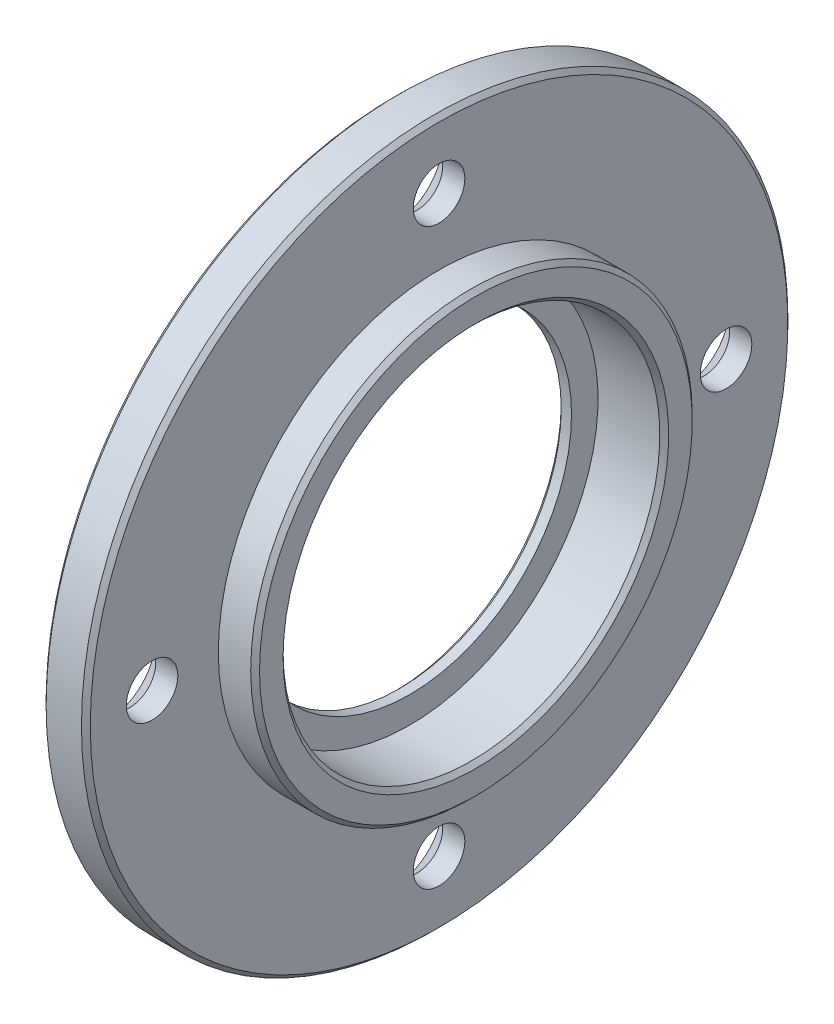
from build123d import *

# Parameters (mm, degrees)
SKETCH2_R          = 1.75
CUT_EXTRUDE1_DEPTH = 3
CHAMFER1_SIZE      = 1.5
CHAMFER2_SIZE      = 0.3


with BuildPart() as part:
    # Sketch1 → Revolve1 (revolve)
    with BuildSketch(Plane.XY, mode=Mode.PRIVATE) as revolve1_sk:
        Polygon((0, 11), (0, 24), (3, 24), (3, 15), (5.5, 15), (5.5, 12.8), (1, 12.8), (1, 11), align=None)
    revolve(revolve1_sk.sketch.rotate(Axis((0, 0, 0), (1, 0, 0)), 90), axis=Axis((0, 0, 0), (1, 0, 0)))

    # Sketch2 → Cut-Extrude1 (cut)
    with BuildSketch(Plane(origin=(3, 0, 0), x_dir=(0, 0, -1), z_dir=(1, 0, 0))):
        with Locations((0, 19.5)):
            Circle(SKETCH2_R)
        with Locations((19.5, 0)):
            Circle(SKETCH2_R)
        with Locations((0, -19.5)):
            Circle(SKETCH2_R)
        with Locations((-19.5, 0)):
            Circle(SKETCH2_R)
    extrude(amount=-CUT_EXTRUDE1_DEPTH, mode=Mode.SUBTRACT)

    # Chamfer1
    chamfer1_edges = [part.edges().sort_by_distance(p)[0] for p in [
        (0, 19.5, 1.75),
        (0, 0, -17.75),
        (0, -19.5, 1.75),
        (0, 0, 21.25),
    ]]
    chamfer(chamfer1_edges, length=CHAMFER1_SIZE)

    # Chamfer2
    chamfer2_edges = [part.edges().sort_by_distance(p)[0] for p in [
        (3, 0, -24),
        (0, 0, -24),
        (0, 0, -11),
        (5.5, 0, -12.8),
        (5.5, 0, -15),
    ]]
    chamfer(chamfer2_edges, length=CHAMFER2_SIZE)


solid = part.part
